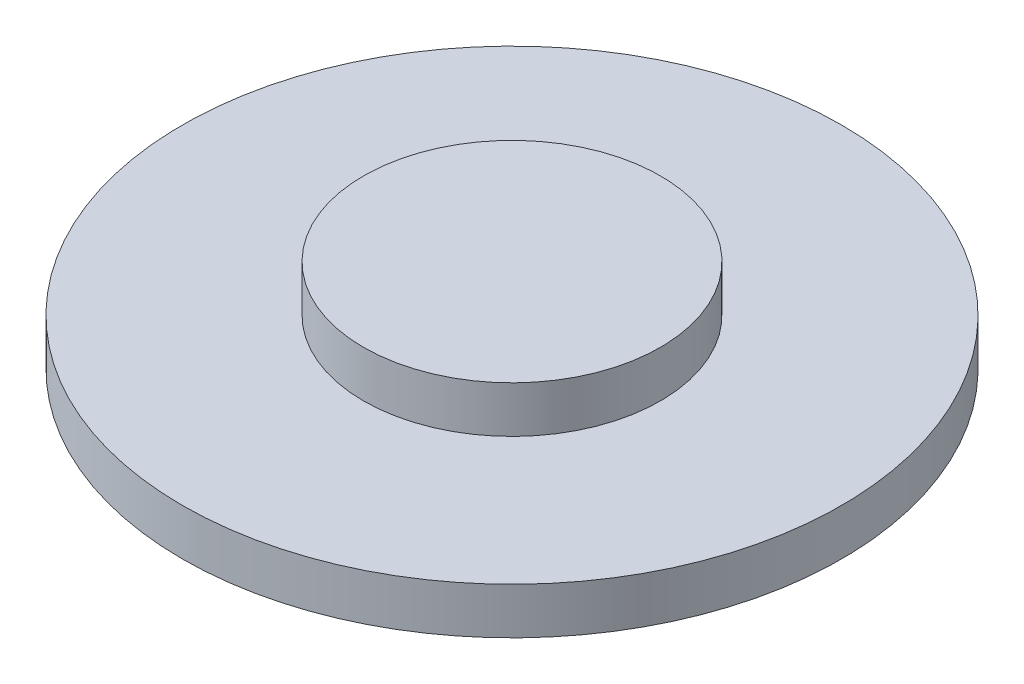
SolidWorks part; units mm, degrees
material "S45C"
ref_plane "Front Plane" through (0, 0, 0) normal (0, 0, 1) x (1, 0, 0)
ref_plane "Top Plane" through (0, 0, 0) normal (0, 1, 0) x (1, 0, 0)
ref_plane "Right Plane" through (0, 0, 0) normal (1, 0, 0) x (0, 0, -1)
sketch "Sketch1" plane through (0, 0, 0) normal (0, 1, 0) x (1, 0, 0)
  circle A0 centre (0, 0) radius 35.5
  dimension "D1" = 71
extrude "Boss-Extrude1" add sketch "Sketch1" along normal blind 5
sketch "Sketch2" plane through (0, 5, 0) normal (0, 1, 0) x (1, 0, 0)
  circle A0 centre (0, 0) radius 15.9958
extrude "Boss-Extrude2" add sketch "Sketch2" along normal blind 5
